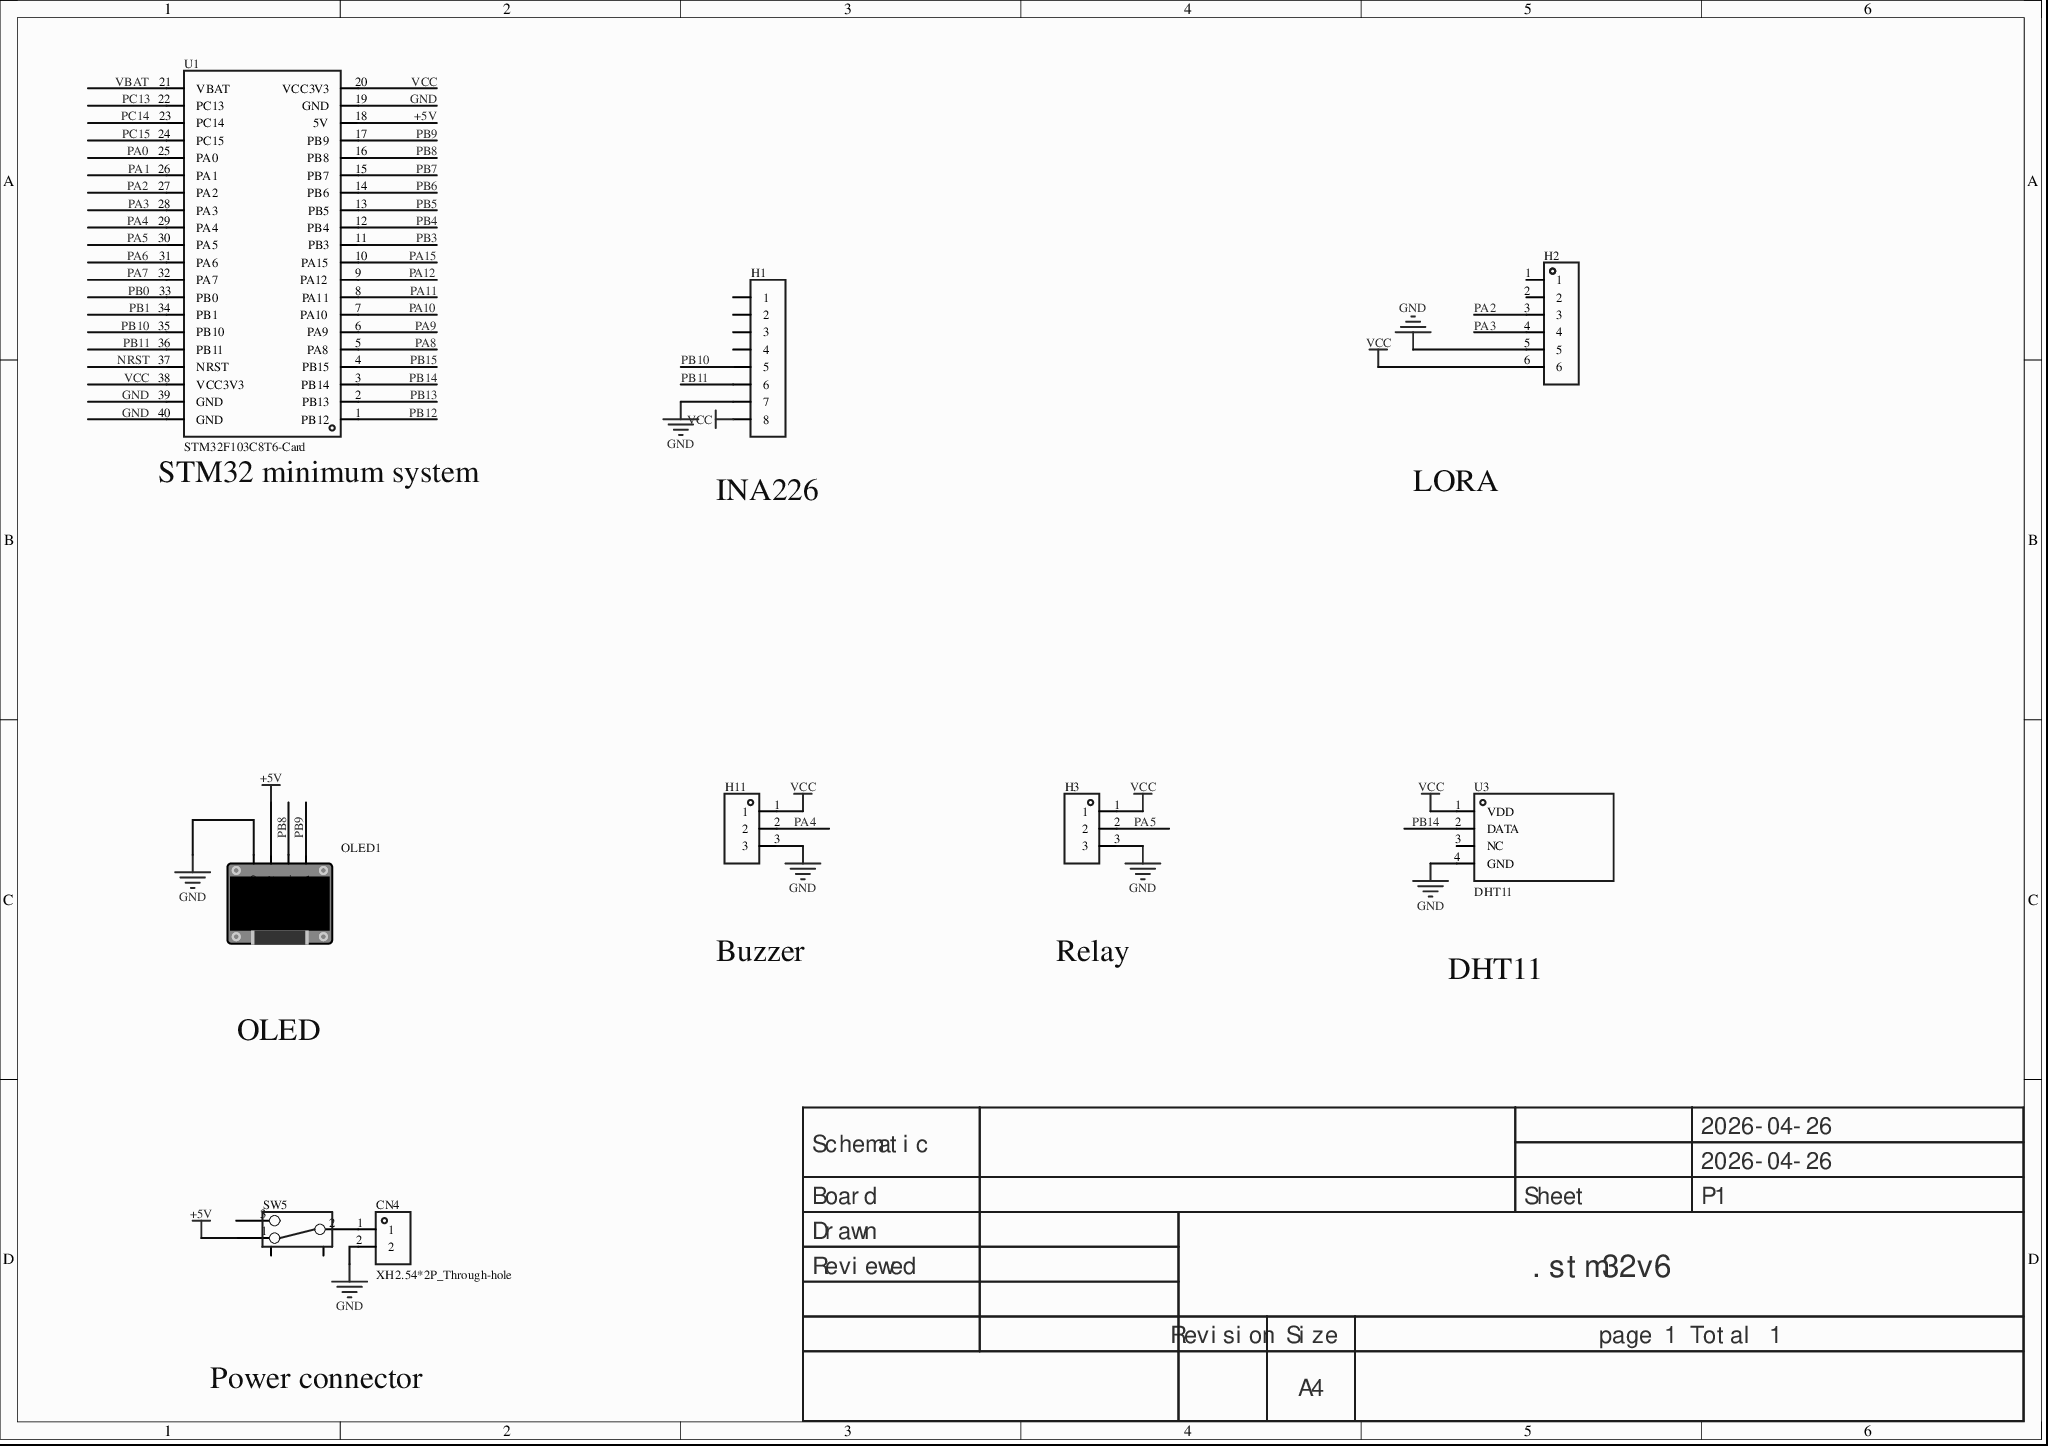
[diagram p0: MISC51756-3.schdoc]
# Altium project MISC51756-2.PrjPcb
1 sheet, 9 parts. Net scope: global (net labels, ports and power ports of the same name join across sheets).
Board file: MISC51756.pcbdoc

## Sheet MISC51756-3.schdoc
size 297 x 209 mm; Version: V1.0; @Project Name: MISC51756; @Page Count: 1; @Update Date: 2026-04-26; @Create Date: 2026-04-26; @Schematic Name: MISC51756; @Page No: 1; @Create Time: 23:22:16; @Update Time: 17:32:40; @Board Name: MISC51756

### Parts
CN4  XH2.54*2P_Through-hole  [CONN-TH_2P-P2.50-XH2.54-2P]
H1  (no value)  [HDR-TH_8P-P2.54-V-F-1]
H2  (no value)  [HDR-TH_6P-P2.54-V-F]
H3  (no value)  [HDR-TH_3P-P2.54-V-F]
H11  (no value)  [HDR-TH_3P-P2.54-V-F]
OLED1  (no value)  [0.96OLED_4P]
SW5  (no value)  [拨动开关]
U1  STM32F103C8T6-Card  [CONN-TH_L53.3-W22.9_STM32F103C8T6-CARD]
U3  DHT11  [SENSOR-TH_DHT11]

### Nets
+5V: OLED1.2(VCC) SW5.1 U1.18(5V)
GND: CN4.2 H1.7 H2.5 H3.3 H11.3 OLED1.1(GND) U1.19(GND) U1.39(GND) U1.40(GND) U3.4(GND)
VCC: H1.8 H2.6 H3.1 H11.1 U1.20(VCC3V3) U1.38(VCC3V3) U3.1(VDD)
NRST: U1.37(NRST)
PA0: U1.25(PA0)
PA1: U1.26(PA1)
PA2: H2.3 U1.27(PA2)
PA3: H2.4 U1.28(PA3)
PA4: H11.2 U1.29(PA4)
PA5: H3.2 U1.30(PA5)
PA6: U1.31(PA6)
PA7: U1.32(PA7)
PA8: U1.5(PA8)
PA9: U1.6(PA9)
PA10: U1.7(PA10)
PA11: U1.8(PA11)
PA12: U1.9(PA12)
PA15: U1.10(PA15)
PB0: U1.33(PB0)
PB1: U1.34(PB1)
PB3: U1.11(PB3)
PB4: U1.12(PB4)
PB5: U1.13(PB5)
PB6: U1.14(PB6)
PB7: U1.15(PB7)
PB8: OLED1.3(SCL) U1.16(PB8)
PB9: OLED1.4(SDA) U1.17(PB9)
PB10: H1.5 U1.35(PB10)
PB11: H1.6 U1.36(PB11)
PB12: U1.1(PB12)
PB13: U1.2(PB13)
PB14: U1.3(PB14) U3.2(DATA)
PB15: U1.4(PB15)
PC13: U1.22(PC13)
PC14: U1.23(PC14)
PC15: U1.24(PC15)
VBAT: U1.21(VBAT)
NetCN4_1: CN4.1 SW5.2

Not connected (* = marked no-connect by the designer): H1 1 2 3 4; H2 1 2; SW5 3 4 5; U3 3(NC)

### Notes on the sheet
- (near U1) STM32 minimum system
- (near H1) INA226
- LORA
- OLED
- Buzzer
- Relay
- DHT11
- Power connector
- Labels drawn without touching a wire or pin: VCC
- 2026-04-26
- Schematic
- Board
- Sheet
- P1
- Drawn
- Reviewed
- .stm32v6
- Revision
- Size
- A4
- page 1 Total 1

### Library data of the parts
CN4 = XH2.54*2P_直插: 3D Model: 325c595e30db4df8abe76612dd40b0fa0819f05c4eef4c71ace90d822a990e87; 3D Model Transform: 295.275,228.346,0,180,0,0,-0.002,-20.079,-137.795; AddInBom: yes; Symbol: XH2.54*2P_Through-hole; Device: XH2.54*2P_Through-hole; LCSC Part Name: XH2.54*2P_直插; Supplier Part: C9900008615; Manufacturer Part: XH2.54*2P_直插; Supplier Footprint: XH2.54_2P; JLCPCB Part Class: Extended Part; Supplier: LCSC; FootprintName: CONN-TH_2P-P2.50-XH2.54-2P; ConvertToPcb: yes; ModelName: CONN-TH_2P-P2.50-XH2.54-2P
H1 = HDR-F_2.54_1x8P: Symbol: Header-Female-2.54_1x8; AddInBom: yes; ModelId: 0f7e4d9227ef4fa08d5469c22cc70cdb; ModelName: HDR-F-2.54_1x8; ModelTransform: 799.99844,100,0,0,0,0,0,0,-118.11; Device: HDR-F_2.54_1x8P; ConvertToPcb: yes; FootprintName: HDR-TH_8P-P2.54-V-F-1; SupplierPart: C27438; Supplier Footprint: 插件
H2 = HDR-F_2.54_1x6P: Symbol: Header-Female-2.54_1x6; ConvertToPcb: yes; ModelId: 0f5bcf94dcda47d085f24cdca1696fe9; ModelTransform: 619.684,94.488,0,0,0,0,0,0,-125.984; Device: HDR-F_2.54_1x6P; AddInBom: yes; SupplierPart: C40877; Supplier Footprint: 插件; FootprintName: HDR-TH_6P-P2.54-V-F; ModelName: HDR-TH_6P-P2.54-V-F
H3 H11 = HDR-F_2.54_1x3P: Symbol: PM254V-11-03-H85; 3D Model: f3b3cc5aae9641bf9e56fc160cef875b; 3D Model Transform: 299.9994,100,0,0,0,0,0,0,-118.11; ConvertToPcb: yes; ModelName: HDR2.54-F-LI-1X3P; Device: HDR-F_2.54_1x3P; Supplier Part: C541850; Supplier Footprint: 插件; AddInBom: yes; FootprintName: HDR-TH_3P-P2.54-V-F
OLED1 = 0.96OLED模块_4P: Symbol: 0.96OLED module_4P; ConvertToPcb: yes; ModelId: 79c000fdb68d45a296c2e9bedf4f9055; ModelTransform: 1393.69792,1318.895,0,0,0,0,0,-560.079,-137.795; Device: 0.96OLED module_4P; AddInBom: yes; FootprintName: 0.96OLED_4P; Supplier Footprint: 插件; ModelName: 0.96OLED_4P
SW5 = 拨动开关_正: Symbol: Toggle switch; Device: Toggle switch_positive; 3D Model: 4321fe59a4074cbfb4989553f297c68f0819f05c4eef4c71ace90d822a990e87; 3D Model Transform: 370.09,208.7,472.35,0,0,0,0,0,-110; ConvertToPcb: yes; ModelName: SW-TH_SS-12D02-VG4; Supplier Footprint: 插件; FootprintName: Toggle switch; AddInBom: yes
U1 = STM32F103C8T6-Card: AddInBom: yes; Symbol: STM32F103C8T6-CARD; Device: STM32F103C8T6-Card; LCSC Part Name: STM32F103C8T6-Card; SupplierPart: C9900077949; ManufacturerPart: STM32F103C8T6-Card; Supplier Footprint: 插件; Supplier: LCSC; ConvertToPcb: yes; FootprintName: CONN-TH_L53.3-W22.9_STM32F103C8T6-CARD
U3 = DHT11: New capacitive digital temperature and humidity sensor; old model discontinued 16.1x12.6x5.8mm; Manufacturer: 广州奥松; AddInBom: yes; ModelId: 6dde47d4d8bf4fa598dffcc067449c1d; ModelTransform: 236.25937,492.125,0,270,0,0,0,-11.811,-196.85; Symbol: DHT11; Device: DHT11; LCSC Part Name: 新款电容式数字温湿度传感器,老款已停产16.1x12.6x5.8mm DHT11  电容式传感器; SupplierPart: C117051; ManufacturerPart: DHT11; Supplier Footprint: SIP-4; JLCPCB Part Class: Extended library; Datasheet: https://atta.szlcsc.com/upload/public/pdf/source/20170703/1499081238365.pdf; Supplier: LCSC; ConvertToPcb: yes; FootprintName: SENSOR-TH_DHT11; ModelName: SENSOR-TH_DHT11